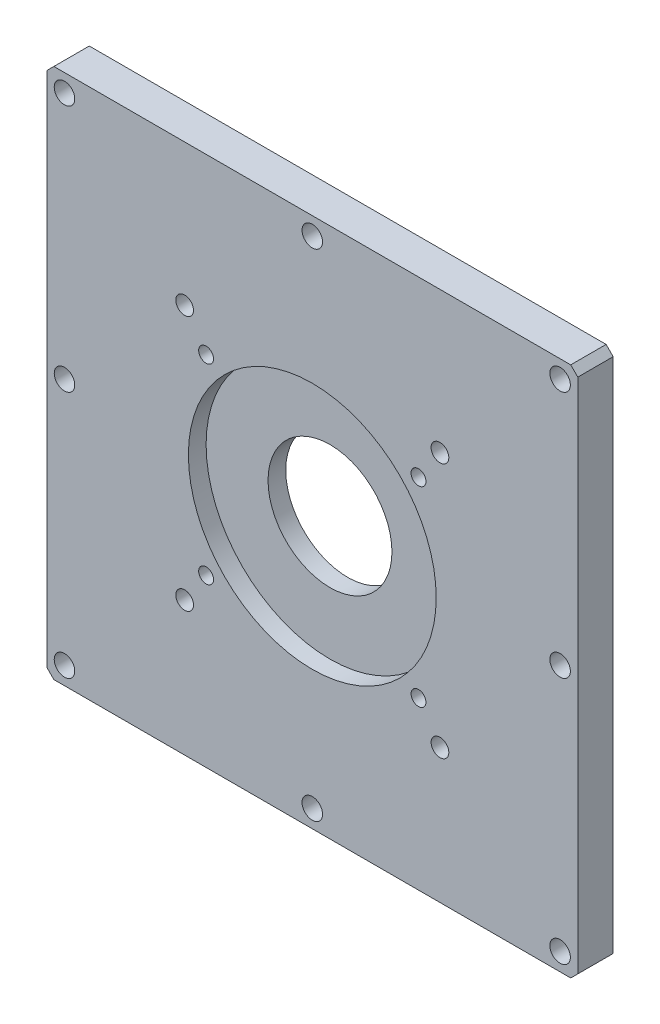
from build123d import *

# Parameters (mm, degrees)
SKETCH_1_W             = 150
SKETCH_1_H             = 150
EXTRUDE_1_DEPTH        = 5
SKETCH_3_R             = 17.5
CUT_EXTRUDE_1_DEPTH    = 107.536378763
HOLE_WIZARD_M5_1_D     = 5.8
CHAMFER_1_SIZE         = 2
SKETCH_6_R             = 35
CUT_EXTRUDE_2_DEPTH    = 5
HOLE_WIZARD_M6_1_D     = 5
HOLE_WIZARD_M6_1_DEPTH = 10
HOLE_WIZARD_M5_1_2_D   = 4.2


with BuildPart() as part:
    # 草图1 → 凸台-拉伸1 (new, symmetric)
    with BuildSketch(Plane.XY):
        Rectangle(SKETCH_1_W, SKETCH_1_H)
    extrude(amount=EXTRUDE_1_DEPTH, both=True)

    # 草图3 → 切除-拉伸1 (cut, through all)
    with BuildSketch(Plane(origin=(0, 0, -5), x_dir=(-1, 0, 0), z_dir=(0, 0, -1))):
        with Locations((0, -1)):
            Circle(SKETCH_3_R)
    extrude(amount=-CUT_EXTRUDE_1_DEPTH, mode=Mode.SUBTRACT)

    # Hole Wizard M5 _1 (through all)
    with Locations(Plane(origin=(0, 0, -5), x_dir=(-1, 0, 0), z_dir=(0, 0, -1))):
        with Locations((-70, 70), (-70, 0), (-70, -70), (0, -70), (70, -70), (70, 0), (70, 70), (0, 70)):
            Hole(HOLE_WIZARD_M5_1_D / 2)

    # 倒角1
    chamfer_1_edges = [part.edges().sort_by_distance(p)[0] for p in [
        (75, -75, 0),
        (-75, -75, 0),
        (-75, 75, 0),
        (75, 75, 0),
    ]]
    chamfer(chamfer_1_edges, length=CHAMFER_1_SIZE)

    # 草图6 → 切除-拉伸2 (cut)
    with BuildSketch(Plane.XY.offset(5)):
        with Locations((0, -1)):
            Circle(SKETCH_6_R)
    extrude(amount=-CUT_EXTRUDE_2_DEPTH, mode=Mode.SUBTRACT)

    # M6 螺纹孔1
    with Locations(Plane.XY.offset(5)):
        with Locations((-36.06, 35.06), (0, -1), (36.06, -37.06), (36.06, 35.06), (-36.06, -37.06)):
            Hole(HOLE_WIZARD_M6_1_D / 2, depth=HOLE_WIZARD_M6_1_DEPTH)

    # Hole Wizard M5 _1 2 (through all)
    with Locations(Plane(origin=(0, 0, -5), x_dir=(-1, 0, 0), z_dir=(0, 0, -1))):
        with Locations((-30, 26), (30, 26), (-30, -28), (30, -28)):
            Hole(HOLE_WIZARD_M5_1_2_D / 2)


solid = part.part
